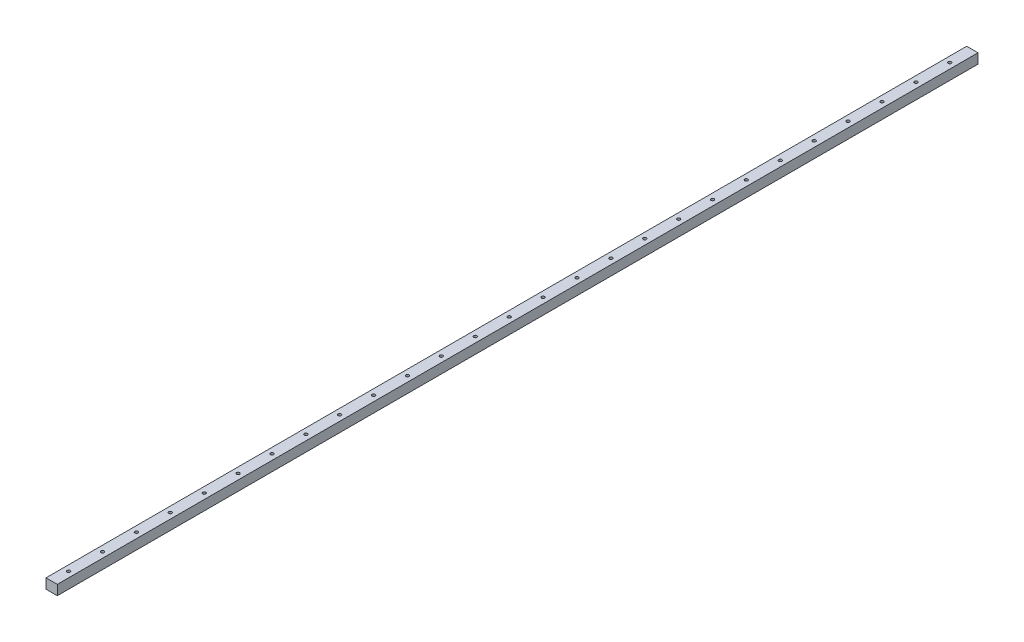
from build123d import *

# Parameters (mm, degrees)
SKETCH_1_W                = 20
SKETCH_1_H                = 17.5
EXTRUDE_1_DEPTH           = 1630
HOLE_WIZARD_1_D           = 5.5
HOLE_WIZARD_1_CBORE_D     = 10
HOLE_WIZARD_1_CBORE_DEPTH = 5.7
PATTERN_LINEAR_1_COUNT    = 27
PATTERN_LINEAR_1_PITCH    = 60


with BuildPart() as part:
    # 草图1 → 凸台-拉伸1 (new body)
    with BuildSketch(Plane.XY):
        with Locations((10, 8.75)):
            Rectangle(SKETCH_1_W, SKETCH_1_H)
    extrude(amount=EXTRUDE_1_DEPTH)

    # 打孔尺寸(%根据)内六角圆柱头螺钉的类型1 (through all)
    with Locations(Plane(origin=(0, 0, 0), x_dir=(-1, 0, 0), z_dir=(0, -1, 0))):
        with Locations((-10, -1600)):
            hole_wizard_1 = CounterBoreHole(HOLE_WIZARD_1_D / 2, HOLE_WIZARD_1_CBORE_D / 2, HOLE_WIZARD_1_CBORE_DEPTH)

    # 阵列(线性)1: 打孔尺寸(%根据)内六角圆柱头螺钉的类型1 ×27
    with Locations(*[(0, 0, -i * PATTERN_LINEAR_1_PITCH) for i in range(1, PATTERN_LINEAR_1_COUNT)]):
        add(hole_wizard_1, mode=Mode.SUBTRACT)


solid = part.part
